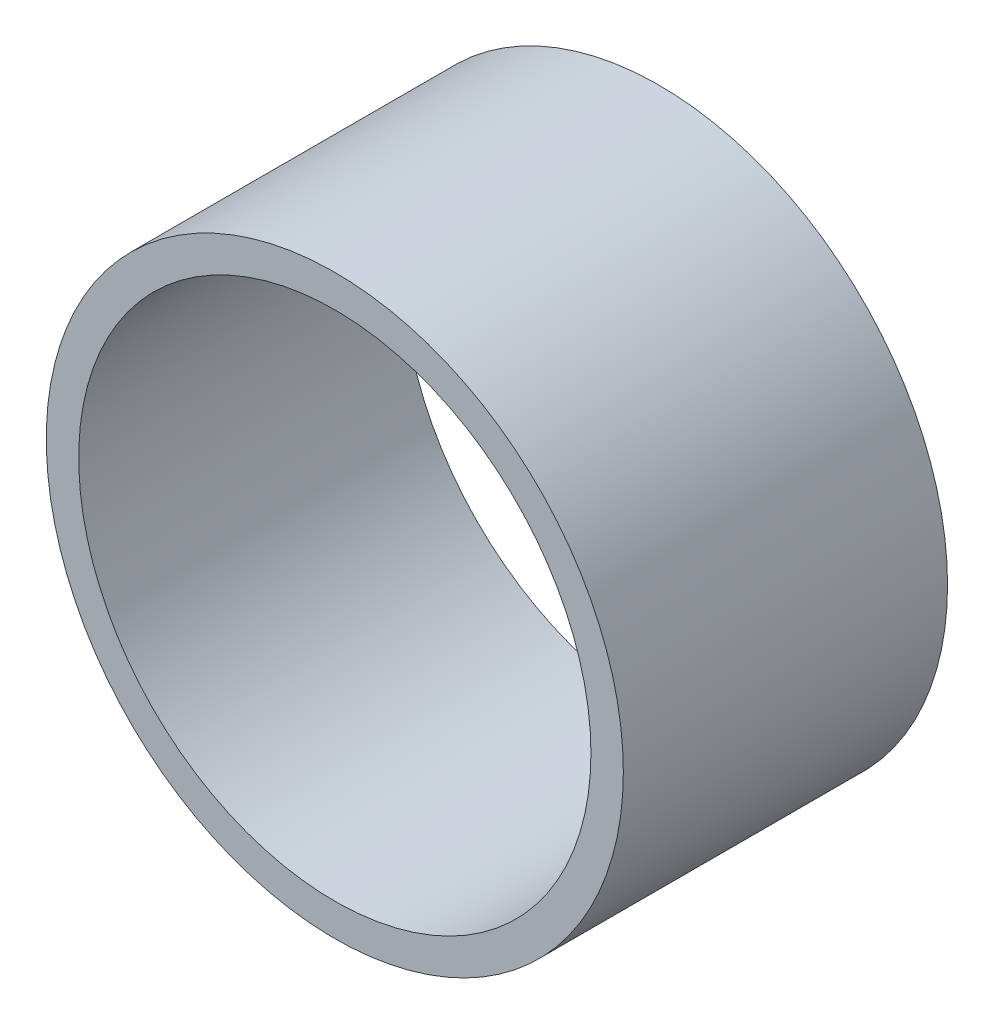
SolidWorks part; units mm, degrees
material "Q235B"
ref_plane "Front Plane" through (0, 0, 0) normal (0, 0, 1) x (1, 0, 0)
ref_plane "Top Plane" through (0, 0, 0) normal (0, 1, 0) x (1, 0, 0)
ref_plane "Right Plane" through (0, 0, 0) normal (1, 0, 0) x (0, 0, -1)
other "Configuration Table"
sketch "Sketch1" plane through (0, 0, 0) normal (0, 0, 1) x (1, 0, 0)
  circle A0 centre (0, 0) radius 44.5
  circle A1 centre (0, 0) radius 39.5
  dimension "D1" = 89
  dimension "D2" = 79
extrude "Boss-Extrude1" add sketch "Sketch1" along normal blind 50
